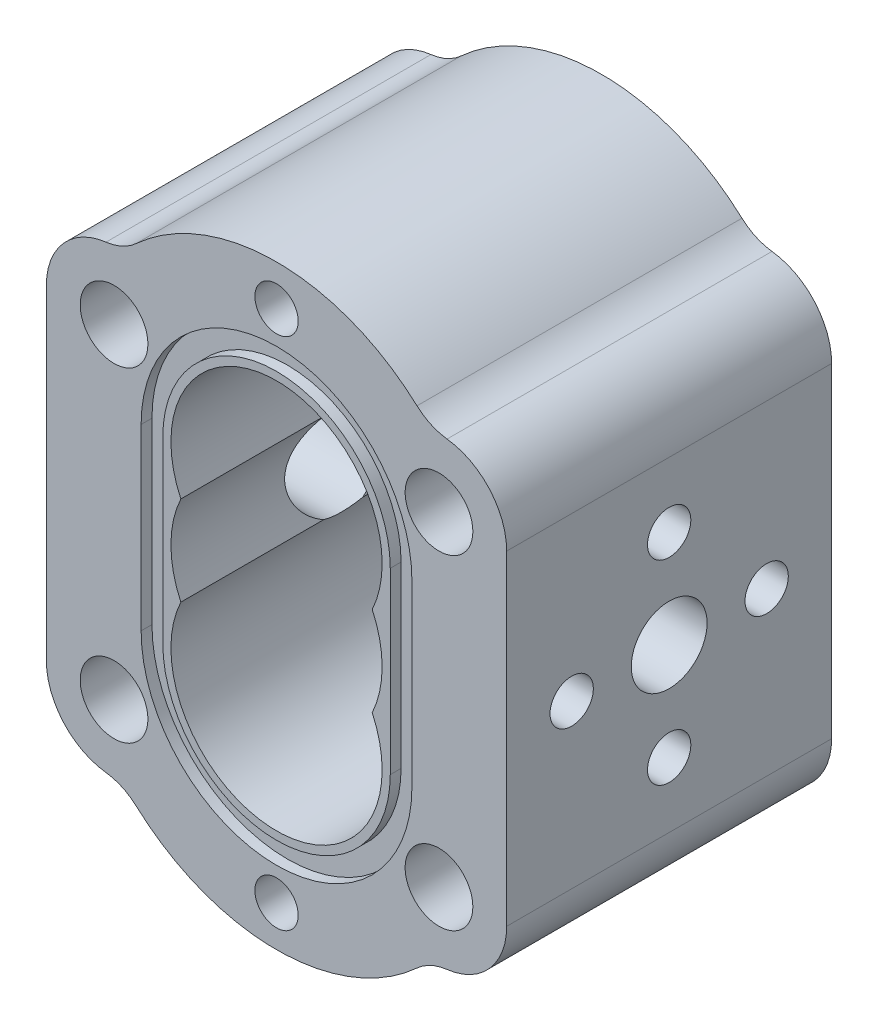
from build123d import *

# Parameters (mm, degrees)
EXTRUDE_1_DEPTH          = 60
SKETCH_3_R               = 6.25
CUT_EXTRUDE_1_DEPTH      = 92.821838361
CUT_EXTRUDE_2_DEPTH      = 92.821838361
CUT_EXTRUDE_3_DEPTH      = 2
SKETCH_6_R               = 4
CUT_EXTRUDE_4_DEPTH      = 6
CUT_EXTRUDE_5_REACH      = 120.048
CUT_EXTRUDE_5_END_RADIUS = 19.5
SKETCH_10_R              = 7
CUT_EXTRUDE_6_REACH      = 120.048
SKETCH_11_R              = 9
SKETCH_7_R               = 4
CUT_EXTRUDE_7_DEPTH      = 15
FILLET_1_R               = 10


with BuildPart() as part:
    # 草图2 → 凸台-拉伸1 (new body)
    with BuildSketch(Plane.XY):
        with BuildLine():
            Line((-42.5, 30), (-42.5, -30))
            ThreePointArc((-42.5, -30), (-38.283749789, -39.36106241), (-28.479281689, -42.407151801))
            ThreePointArc((-28.479281689, -42.407151801), (0, -55), (28.479281689, -42.407151801))
            ThreePointArc((28.479281689, -42.407151801), (38.283749789, -39.36106241), (42.5, -30))
            Line((42.5, -30), (42.5, 30))
            ThreePointArc((42.5, 30), (38.283749789, 39.36106241), (28.479281689, 42.407151801))
            ThreePointArc((28.479281689, 42.407151801), (0, 55), (-28.479281689, 42.407151801))
            ThreePointArc((-28.479281689, 42.407151801), (-38.283749789, 39.36106241), (-42.5, 30))
        make_face()
    extrude(amount=EXTRUDE_1_DEPTH)

    # 草图3 → 切除-拉伸1 (cut, through all)
    with BuildSketch(Plane.XY.offset(60)):
        with Locations((-30, 30)):
            Circle(SKETCH_3_R)
        with Locations((30, 30)):
            Circle(SKETCH_3_R)
        with Locations((-30, -30)):
            Circle(SKETCH_3_R)
        with Locations((30, -30)):
            Circle(SKETCH_3_R)
    extrude(amount=-CUT_EXTRUDE_1_DEPTH, mode=Mode.SUBTRACT)

    # 草图4 → 切除-拉伸2 (cut, through all)
    with BuildSketch(Plane.XY.offset(60)):
        with BuildLine():
            ThreePointArc((17.668828484, 8.25), (0, 36), (-17.668828484, 8.25))
            ThreePointArc((-17.668828484, 8.25), (-19.5, 0), (-17.668828484, -8.25))
            ThreePointArc((-17.668828484, -8.25), (0, -36), (17.668828484, -8.25))
            ThreePointArc((17.668828484, -8.25), (19.5, 0), (17.668828484, 8.25))
        make_face()
    extrude(amount=-CUT_EXTRUDE_2_DEPTH, mode=Mode.SUBTRACT)

    # 草图5 → 切除-拉伸3 (cut)
    with BuildSketch(Plane.XY.offset(60)):
        with BuildLine():
            Line((-25, 16.5), (-25, -16.5))
            ThreePointArc((-25, -16.5), (0, -41.5), (25, -16.5))
            Line((25, -16.5), (25, 16.5))
            ThreePointArc((25, 16.5), (0, 41.5), (-25, 16.5))
        make_face()
        with BuildLine():
            Line((-21, 16.5), (-21, -16.5))
            ThreePointArc((-21, -16.5), (0, -37.5), (21, -16.5))
            Line((21, -16.5), (21, 16.5))
            ThreePointArc((21, 16.5), (0, 37.5), (-21, 16.5))
        make_face(mode=Mode.SUBTRACT)
    cut_extrude_3 = extrude(amount=-CUT_EXTRUDE_3_DEPTH, mode=Mode.SUBTRACT)

    # 草图6 → 切除-拉伸4 (cut)
    with BuildSketch(Plane.XY.offset(60)):
        with Locations((0, 47.5)):
            Circle(SKETCH_6_R)
        with Locations((0, -47.5)):
            Circle(SKETCH_6_R)
    extrude(amount=-CUT_EXTRUDE_4_DEPTH, mode=Mode.SUBTRACT)

    # 镜向1: 切除-拉伸3 across plane
    add(cut_extrude_3.mirror(Plane.XY.offset(30)), mode=Mode.SUBTRACT)

    # 切除-拉伸5: up to this cylinder (the profile starts outside it)
    cut_extrude_5_end = Plane(origin=(0, 0, 30), z_dir=(0, 0, 1)) * Cylinder(CUT_EXTRUDE_5_END_RADIUS, 280.096, mode=Mode.PRIVATE)
    # 草图10 → 切除-拉伸5 (cut, up to the surface)
    with BuildSketch(Plane(origin=(43, 0, 0), x_dir=(0, 0, -1), z_dir=(1, 0, 0)), mode=Mode.PRIVATE) as cut_extrude_5_sk1:
        with Locations(Location((-30, 0, 0), (0, 0, 90))):
            Circle(SKETCH_10_R)
    cut_extrude_5_tool1 = extrude(cut_extrude_5_sk1.sketch, amount=-CUT_EXTRUDE_5_REACH, mode=Mode.PRIVATE) - cut_extrude_5_end
    add(cut_extrude_5_tool1.solids().sort_by_distance((43, 0, 30))[0], mode=Mode.SUBTRACT)

    # 草图11 → 切除-拉伸6 (cut, up to next)
    with BuildSketch(Plane.ZY.offset(43), mode=Mode.PRIVATE) as cut_extrude_6_sk1:
        with Locations(Location((30, 0, 0), (0, 0, 246.443535691))):
            Circle(SKETCH_11_R)
    cut_extrude_6_tool1 = extrude(cut_extrude_6_sk1.sketch, amount=-CUT_EXTRUDE_6_REACH, mode=Mode.PRIVATE) & part.part
    add(cut_extrude_6_tool1.solids().sort_by_distance((-43, 0, 30))[0], mode=Mode.SUBTRACT)

    # 草图7 → 切除-拉伸7 (cut)
    with BuildSketch(Plane(origin=(43, 0, 0), x_dir=(0, 0, -1), z_dir=(1, 0, 0))):
        with Locations(Location((-30, 18, 0), (0, 0, 90))):
            Circle(SKETCH_7_R)
        with Locations(Location((-48, 0, 0), (0, 0, 90))):
            Circle(SKETCH_7_R)
        with Locations(Location((-30, -18, 0), (0, 0, 90))):
            Circle(SKETCH_7_R)
        with Locations(Location((-12, 0, 0), (0, 0, 90))):
            Circle(SKETCH_7_R)
    cut_extrude_7 = extrude(amount=-CUT_EXTRUDE_7_DEPTH, mode=Mode.SUBTRACT)

    # 镜向2: 切除-拉伸7 across plane
    add(cut_extrude_7.mirror(Plane(origin=(0, 0, 0), x_dir=(0, 0, 1), z_dir=(1, 0, 0))), mode=Mode.SUBTRACT)

    # 圆角1
    fillet_1_edges = [part.edges().sort_by_distance(p)[0] for p in [
        (-28.479281689, 42.407151801, 30),
        (28.479281689, 42.407151801, 30),
        (28.479281689, -42.407151801, 30),
        (-28.479281689, -42.407151801, 30),
    ]]
    fillet(fillet_1_edges, radius=FILLET_1_R)


solid = part.part
